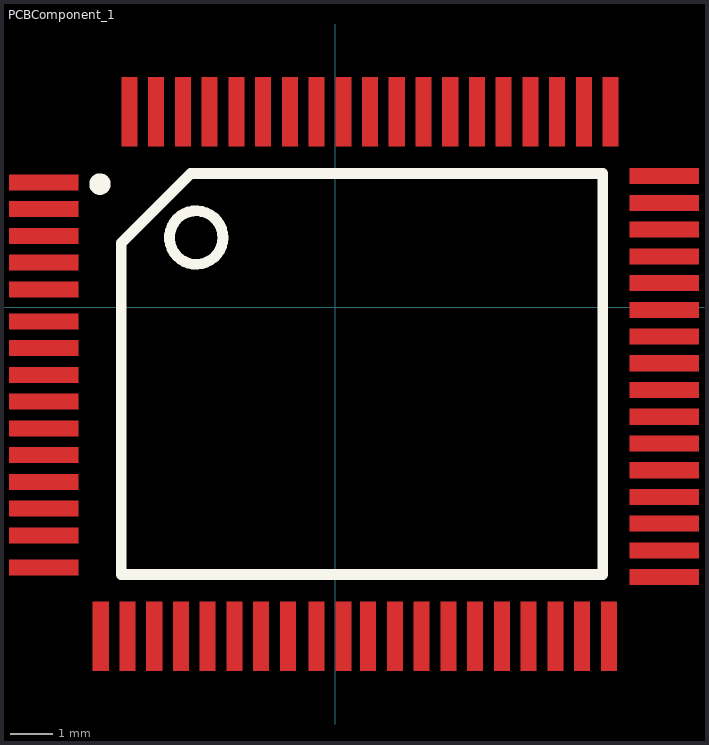
[diagram p0: the footprint, top view; thin cyan lines are the x and y axes]
# Altium footprint library MISC82341-17.PcbLib: 1 footprints
Each footprint in its own frame and in the unit in brackets; x right, y up, seen from the top. Pads: shape width x height; smd on the part's side, far side on the other; paste and mask are expansions set on the pad; w line width, h text height; cw(c..) or ccw(c..) is an arc to the next point about the centre after c.

## PCBComponent_1 [mm]
Top Layer:
  region: -6.095,-6.373 -6.095,-5.992 -7.746,-5.992 -7.746,-6.373
  region: -6.095,-5.611 -6.095,-5.23 -7.746,-5.23 -7.746,-5.611
  region: -6.095,-4.976 -6.095,-4.595 -7.746,-4.595 -7.746,-4.976
  region: -6.095,-4.341 -6.095,-3.96 -7.746,-3.96 -7.746,-4.341
  region: -6.095,-3.706 -6.095,-3.325 -7.746,-3.325 -7.746,-3.706
  region: -6.095,-3.071 -6.095,-2.69 -7.746,-2.69 -7.746,-3.071
  region: -6.095,-2.436 -6.095,-2.055 -7.746,-2.055 -7.746,-2.436
  region: -6.095,-1.801 -6.095,-1.42 -7.746,-1.42 -7.746,-1.801
  region: -6.095,-1.166 -6.095,-0.785 -7.746,-0.785 -7.746,-1.166
  region: -6.095,-0.531 -6.095,-0.15 -7.746,-0.15 -7.746,-0.531
  region: -6.095,0.231 -6.095,0.612 -7.746,0.612 -7.746,0.231
  region: -6.095,0.866 -6.095,1.247 -7.746,1.247 -7.746,0.866
  region: -6.095,1.501 -6.095,1.882 -7.746,1.882 -7.746,1.501
  region: -6.095,2.136 -6.095,2.517 -7.746,2.517 -7.746,2.136
  region: -6.095,2.771 -6.095,3.152 -7.746,3.152 -7.746,2.771
  rectangle: -5.759,-8.638 -5.378,-6.987
  rectangle: -5.124,-8.638 -4.743,-6.987
  rectangle: -4.489,-8.638 -4.108,-6.987
  rectangle: -3.854,-8.638 -3.473,-6.987
  rectangle: -3.219,-8.638 -2.838,-6.987
  rectangle: -2.584,-8.638 -2.203,-6.987
  rectangle: -1.949,-8.638 -1.568,-6.987
  rectangle: -1.314,-8.638 -0.933,-6.987
  rectangle: -0.635,-8.636 -0.254,-6.985
  rectangle: 0,-8.636 0.381,-6.985
  rectangle: 0.591,-8.638 0.972,-6.987
  rectangle: 1.226,-8.638 1.607,-6.987
  rectangle: 1.861,-8.638 2.242,-6.987
  rectangle: 2.496,-8.638 2.877,-6.987
  rectangle: 3.131,-8.638 3.512,-6.987
  rectangle: 3.766,-8.638 4.147,-6.987
  rectangle: 4.401,-8.638 4.782,-6.987
  rectangle: 5.036,-8.638 5.417,-6.987
  rectangle: 5.671,-8.638 6.052,-6.987
  rectangle: 6.306,-8.638 6.687,-6.987
  region: 8.636,-6.604 8.636,-6.223 6.985,-6.223 6.985,-6.604
  region: 8.636,-5.969 8.636,-5.588 6.985,-5.588 6.985,-5.969
  region: 8.636,-5.334 8.636,-4.953 6.985,-4.953 6.985,-5.334
  region: 8.636,-4.699 8.636,-4.318 6.985,-4.318 6.985,-4.699
  region: 8.636,-4.064 8.636,-3.683 6.985,-3.683 6.985,-4.064
  region: 8.636,-3.429 8.636,-3.048 6.985,-3.048 6.985,-3.429
  region: 8.636,-2.794 8.636,-2.413 6.985,-2.413 6.985,-2.794
  region: 8.636,-2.159 8.636,-1.778 6.985,-1.778 6.985,-2.159
  region: 8.636,-1.524 8.636,-1.143 6.985,-1.143 6.985,-1.524
  region: 8.636,-0.889 8.636,-0.508 6.985,-0.508 6.985,-0.889
  region: 8.636,-0.254 8.636,0.127 6.985,0.127 6.985,-0.254
  region: 8.636,0.381 8.636,0.762 6.985,0.762 6.985,0.381
  region: 8.636,1.016 8.636,1.397 6.985,1.397 6.985,1.016
  region: 8.636,1.651 8.636,2.032 6.985,2.032 6.985,1.651
  region: 8.636,2.286 8.636,2.667 6.985,2.667 6.985,2.286
  region: 8.636,2.921 8.636,3.302 6.985,3.302 6.985,2.921
  rectangle: 6.35,3.81 6.731,5.461
  rectangle: 5.715,3.81 6.096,5.461
  rectangle: 5.08,3.81 5.461,5.461
  rectangle: 4.445,3.81 4.826,5.461
  rectangle: 3.81,3.81 4.191,5.461
  rectangle: 3.175,3.81 3.556,5.461
  rectangle: -5.08,3.81 -4.699,5.461
  rectangle: 2.54,3.81 2.921,5.461
  rectangle: -4.445,3.81 -4.064,5.461
  rectangle: 1.905,3.81 2.286,5.461
  rectangle: 1.27,3.81 1.651,5.461
  rectangle: 0.635,3.81 1.016,5.461
  rectangle: 0,3.81 0.381,5.461
  rectangle: -0.635,3.81 -0.254,5.461
  rectangle: -1.905,3.81 -1.524,5.461
  rectangle: -2.54,3.81 -2.159,5.461
  rectangle: -3.175,3.81 -2.794,5.461
  rectangle: -3.81,3.81 -3.429,5.461
  rectangle: -1.27,3.81 -0.889,5.461
  region: 3.683,4.445
Top Overlay:
  circle w0.254: c-3.302,1.651 r0.635
  circle w0.254: c-5.588,2.921 r0.127
  lines w0.254: -5.08,-6.35 6.35,-6.35 6.35,3.175 -3.429,3.175 -5.08,1.524 -5.08,-3.175 -5.08,-6.35